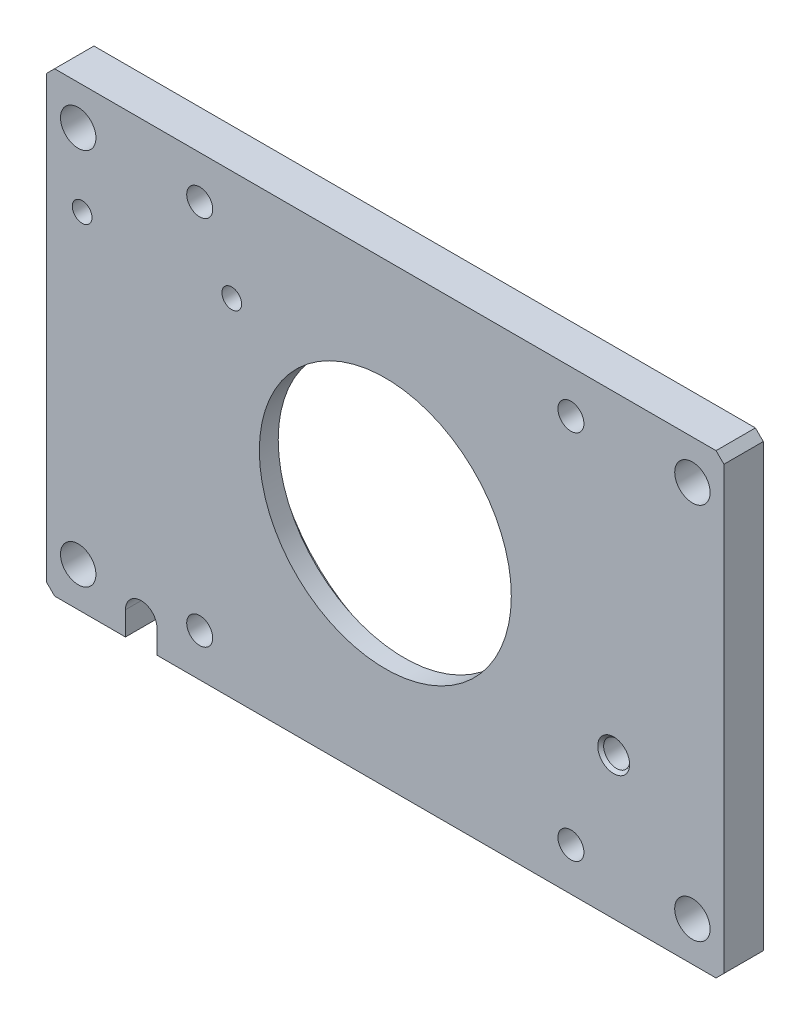
SolidWorks part; units mm, degrees
material "普通碳钢"
ref_plane "前视基准面" through (0, 0, 0) normal (0, 0, 1) x (1, 0, 0)
ref_plane "上视基准面" through (0, 0, 0) normal (0, 1, 0) x (1, 0, 0)
ref_plane "右视基准面" through (0, 0, 0) normal (1, 0, 0) x (0, 0, -1)
sketch "草图1" plane through (0, 0, 0) normal (0, 0, 1) x (1, 0, 0)
  line L1 (-43, 29) -> (43, 29)
  line L2 (-43, 29) -> (-43, -29)
  line L3 (-43, -29) -> (43, -29)
  line L4 (43, 29) -> (43, -29)
  line L5 (-43, 29) -> (43, -29) construction
  line L6 (-43, -29) -> (43, 29) construction
  line L9 (0, 29) -> (0, -29) construction
  line L10 (-43, 0) -> (43, 0) construction
  circle A0 centre (0, 0) radius 16
  circle A1 centre (-39, 24) radius 2.25
  circle A2 centre (39, 24) radius 2.25
  circle A3 centre (39, -24) radius 2.25
  circle A4 centre (-39, -24) radius 2.25
  point P0 (0, 0)
  dimension "D3" = 32
  dimension "D4" = 4.5
  dimension "D6" = 5
  dimension "D1" = 58
  dimension "D2" = 86
  dimension "D5" = 4
extrude "凸台-拉伸1" add sketch "草图1" along normal mid plane 10
hole_wizard "M3 螺纹孔1" positions "草图4" profile "草图3" tap size "M3" standard "GB" end condition through all
sketch "草图4" plane through (0, 0, 5) normal (0, 0, 1) x (1, 0, 0)
  line L0 (-38.5, 15) -> (-19.5, 15) construction
  line L3 (43, 29) -> (-43, 29) construction
  line L4 (-29, 15) -> (-29, 9.6443) construction
  line L7 (-43, 29) -> (-43, -29) construction
  point P0 (-38.5, 15)
  point P2 (-19.5, 15)
  dimension "D1" = 19
  dimension "D2" = 14
  dimension "D3" = 14
sketch "草图3" plane through (-38.5, 15, 5) normal (1, 0, 0) x (0, -1, 0)
  line L0 (0, 0) -> (0, 10)
  line L1 (0, 10) -> (1.25, 10)
  line L2 (1.25, 10) -> (1.25, 0)
  line L5 (1.25, 0) -> (0, 0)
  line L11 (0, -6.35) -> (0, 107.95) construction
  dimension "通孔螺纹孔钻头直径" = 2.5
  dimension "通孔螺纹孔钻头深度" = 10
cosmetic thread "孔螺蚊线1" parameters "D2"=3
cosmetic thread "孔螺蚊线2" parameters "D2"=3
hole_wizard "M4 螺纹孔1" positions "草图6" profile "草图5" tap size "M4" standard "GB" end condition through all
sketch "草图6" plane through (0, 0, 5) normal (0, 0, 1) x (1, 0, 0)
  point P0 (-23.57, 23.57)
  dimension "D1" = 23.57
  dimension "D2" = 23.57
sketch "草图5" plane through (-23.57, 23.57, 5) normal (1, 0, 0) x (0, -1, 0)
  line L0 (0, 0) -> (0, 10)
  line L1 (0, 10) -> (1.65, 10)
  line L2 (1.65, 10) -> (1.65, 0)
  line L5 (1.65, 0) -> (0, 0)
  line L11 (0, -6.35) -> (0, 107.95) construction
  dimension "通孔螺纹孔钻头直径" = 3.3
  dimension "通孔螺纹孔钻头深度" = 10
cosmetic thread "孔螺蚊线3" parameters "D2"=4
mirror "镜向1" about plane through (0, 0, 0) normal (0, 1, 0) of "M4 螺纹孔1"
mirror "镜向2" about plane through (0, 0, 0) normal (1, 0, 0) of "镜向1", "M4 螺纹孔1"
sketch "草图7" plane through (0, 0, 5) normal (0, 0, 1) x (1, 0, 0)
  line L0 (-31, -29) -> (-31, -26) construction
  line L1 (-43, -29) -> (43, -29) construction
  line L2 (-33, -29) -> (-33, -26)
  line L3 (-29, -29) -> (-29, -26)
  line L4 (-43, 29) -> (-43, -29) construction
  arc A0 (-33, -29) -> (-29, -29) centre (-31, -29) ccw
  arc A1 (-29, -26) -> (-33, -26) centre (-31, -26) ccw
  point P4 (-31, -27.5)
  dimension "D1" = 2
  dimension "D2" = 3
  dimension "D3" = 12
extrude "切除-拉伸1" cut sketch "草图7" against normal through all
sketch "草图8" plane through (0, 0, -5) normal (0, 0, -1) x (-1, 0, 0)
  line L1 (-29.3337, 39.5816) -> (30, 39.5816)
  line L2 (-29.3337, 39.5816) -> (-28, -41.6168)
  line L3 (30, -41.6168) -> (-28, -41.6168)
  line L4 (30, 39.5816) -> (30, -41.6168)
  line L5 (43, 29) -> (43, -29) construction
  dimension "D1" = 81.1985
  dimension "D2" = 58
  dimension "D3" = 13
  dimension "D4" = 5.5
extrude "切除-拉伸2" [suppressed] cut sketch "草图8" against normal blind 4 contours L3 L2 L1 L4
sketch "草图9" plane through (0, 0, -5) normal (0, 0, -1) x (-1, 0, 0)
  line L1 (19.0274, 46.0356) -> (-30, 46.0356)
  line L2 (19.0274, 46.0356) -> (19.0274, -41.21)
  line L3 (19.0274, -41.21) -> (-30, -41.21)
  line L4 (-30, 46.0356) -> (-30, -41.21)
  line L5 (19.0274, 46.0356) -> (-30, -41.21) construction
  line L6 (19.0274, -41.21) -> (-30, 46.0356) construction
  point P0 (-5.4863, 2.4128)
  dimension "D1" = 30
extrude "切除-拉伸3" [suppressed] cut sketch "草图9" against normal up to surface (4 mm away)
chamfer "倒角1" distance 1 angle 45 4 edges at (43, -29, 0) (-43, -29, 0) (-43, 29, 0) (43, 29, 0)
sketch "草图10" plane through (0, 29, 0) normal (0, 1, 0) x (1, 0, 0)
  line L1 (160.2117, 17.0468) -> (-56.3387, 17.0468)
  line L2 (160.2117, 17.0468) -> (160.2117, 0)
  line L3 (160.2117, 0) -> (-56.3387, 0)
  line L4 (-56.3387, 17.0468) -> (-56.3387, 0)
  line L5 (160.2117, 17.0468) -> (-56.3387, 0) construction
  line L6 (160.2117, 0) -> (-56.3387, 17.0468) construction
  line L8 (42, 5) -> (-42, 5) construction
  point P0 (51.9365, 8.5234)
  dimension "D1" = 5
extrude "切除-拉伸4" cut sketch "草图10" against normal through all
sketch "草图11" plane through (0, 0, 0) normal (0, 0, -1) x (-1, 0, 0)
  circle A0 centre (0, 0) radius 19.5
  dimension "D1" = 39
extrude "切除-拉伸5" cut sketch "草图11" against normal blind 2.6
hole_wizard "M4 螺纹孔2" positions "3D草图1" profile "草图12" tap size "M4" standard "GB"
sketch3d "3D草图1"
  line L0 (43, -28, 5) -> (43, 28, 5) construction
  point P0 (30.75, -16, 5)
  dimension "D1" = 12.25
  dimension "D2" = 13
sketch "草图12" plane through (30.75, -16, 5) normal (1, 0, 0) x (0, -1, 0)
  line L0 (0, 0) -> (0, 12.4914)
  line L1 (0, 12.4914) -> (1.65, 11.5)
  line L2 (1.65, 11.5) -> (1.65, 0)
  line L5 (1.65, 0) -> (0, 0)
  line L10 (0, 12.4914) -> (-1.65, 11.5) construction
  line L11 (0, -6.35) -> (0, 107.95) construction
  dimension "螺纹孔钻头直径" = 3.3
  dimension "螺纹孔钻头深度" = 11.5
  dimension "导头角度" = 118
cosmetic thread "孔螺蚊线4" [suppressed] parameters "D1"=5, "D2"=4
pattern_linear "阵列(线性)1" [suppressed] count 2 spacing 10
sketch "草图13" plane through (0, 0, 5) normal (0, 0, 1) x (1, 0, 0)
  line L0 (-29, -29) -> (42, -29) construction
  line L1 (43, -28) -> (43, 28) construction
  circle A0 centre (29, -11) radius 1.3504
  dimension "D1" = 18
  dimension "D2" = 14
extrude "切除-拉伸6" cut sketch "草图13" against normal blind 10
hole_wizard "M4 螺纹孔3" positions "3D草图2" profile "草图14" tap size "M4" standard "GB"
sketch3d "3D草图2"
  line L0 (29, -11, 0) -> (29, -11, 5) construction
  point P0 (29, -11, 5)
sketch "草图14" plane through (29, -11, 5) normal (1, 0, 0) x (0, -1, 0)
  line L0 (0, 0) -> (0, 12.4914)
  line L1 (0, 12.4914) -> (1.65, 11.5)
  line L2 (1.65, 11.5) -> (1.65, 0.375)
  line L3 (1.65, 0.375) -> (2.025, 0)
  line L5 (2.025, 0) -> (0, 0)
  line L6 (-1.65, 0.375) -> (-2.025, 0) construction
  line L10 (0, 12.4914) -> (-1.65, 11.5) construction
  line L11 (0, -6.35) -> (0, 107.95) construction
  dimension "螺纹孔钻头直径" = 3.3
  dimension "螺纹孔钻头深度" = 11.5
  dimension "近端锥形沉头孔直径" = 4.05
  dimension "近端锥形沉头孔角度" = 90
  dimension "导头角度" = 118
